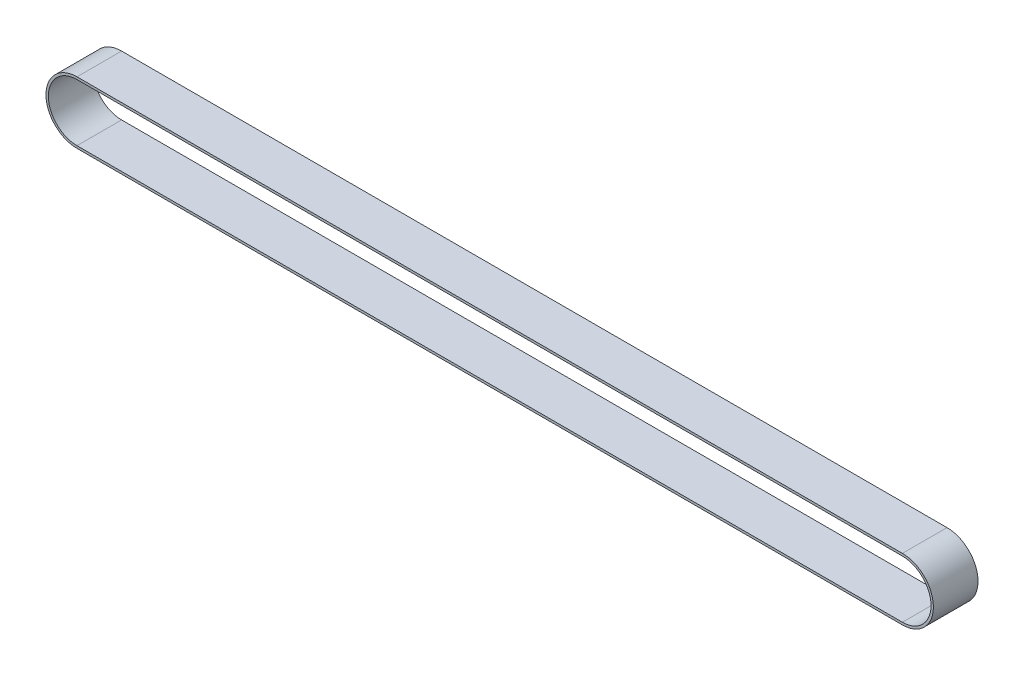
SolidWorks part; units mm, degrees
material "6061 合金"
ref_plane "前视基准面" through (0, 0, 0) normal (0, 0, 1) x (1, 0, 0)
ref_plane "上视基准面" through (0, 0, 0) normal (0, 1, 0) x (1, 0, 0)
ref_plane "右视基准面" through (0, 0, 0) normal (1, 0, 0) x (0, 0, -1)
sketch "草图1" plane through (0, 0, 0) normal (0, 0, 1) x (1, 0, 0)
  line L0 (0, 7.705) -> (222, 7.705)
  line L1 (222, -7.705) -> (0, -7.705)
  line L2 (0, 8.335) -> (222, 8.335)
  line L3 (222, -8.335) -> (0, -8.335)
  arc A0 (0, 7.705) -> (0, -7.705) centre (0, 0) ccw
  arc A1 (222, -7.705) -> (222, 7.705) centre (222, 0) ccw
  arc A2 (222, -8.335) -> (222, 8.335) centre (222, 0) ccw
  arc A3 (0, 8.335) -> (0, -8.335) centre (0, 0) ccw
  dimension "D1" = 15.41
  dimension "D2" = 15.41
  dimension "D3" = 222
  dimension "D4" = 0.63
extrude "凸台-拉伸1" add sketch "草图1" along normal mid plane 12
